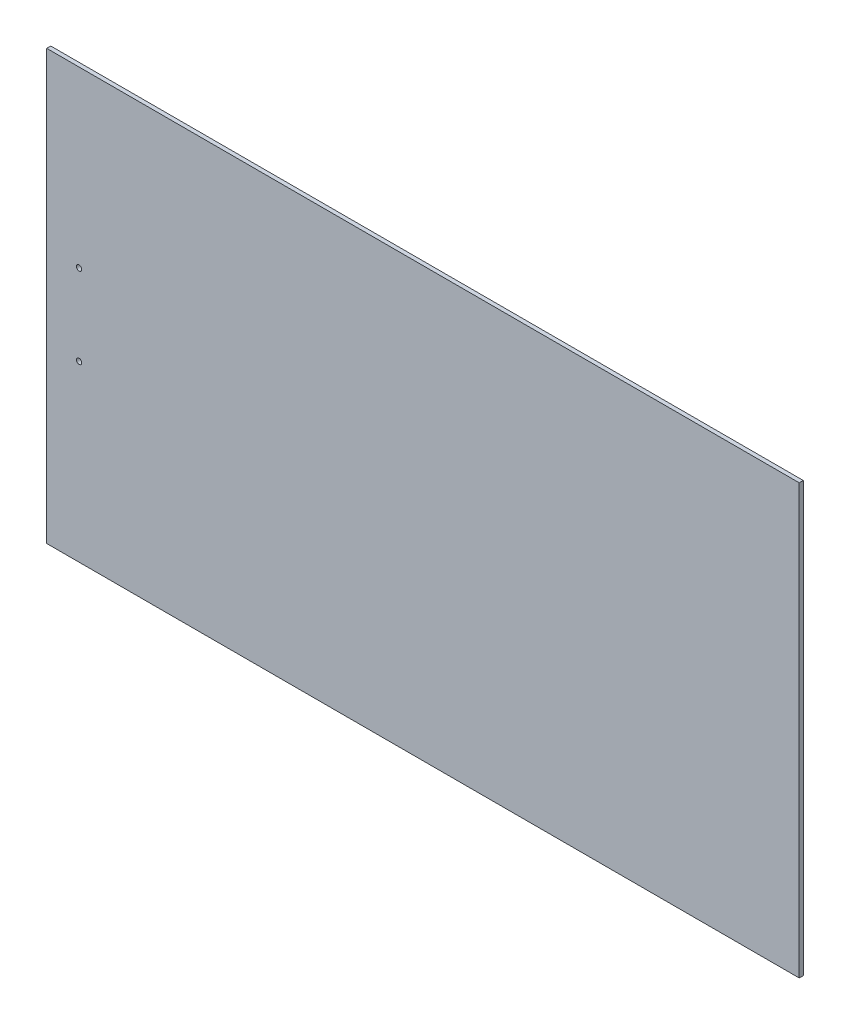
from build123d import *

# Parameters (mm, degrees)
SKETCH_1_W          = 930
SKETCH_1_H          = 530
EXTRUDE_1_DEPTH     = 5
SKETCH_2_R          = 3.3
CUT_EXTRUDE_1_DEPTH = 10


with BuildPart() as part:
    # 草图1 → 凸台-拉伸1 (new body)
    with BuildSketch(Plane.XY):
        Rectangle(SKETCH_1_W, SKETCH_1_H)
    extrude(amount=EXTRUDE_1_DEPTH)

    # 草图2 → 切除-拉伸1 (cut)
    with BuildSketch(Plane(origin=(0, 0, 0), x_dir=(-1, 0, 0), z_dir=(0, 0, -1))):
        with Locations((425, 50)):
            Circle(SKETCH_2_R)
        with Locations((425, -50)):
            Circle(SKETCH_2_R)
    extrude(amount=-CUT_EXTRUDE_1_DEPTH, mode=Mode.SUBTRACT)


solid = part.part
